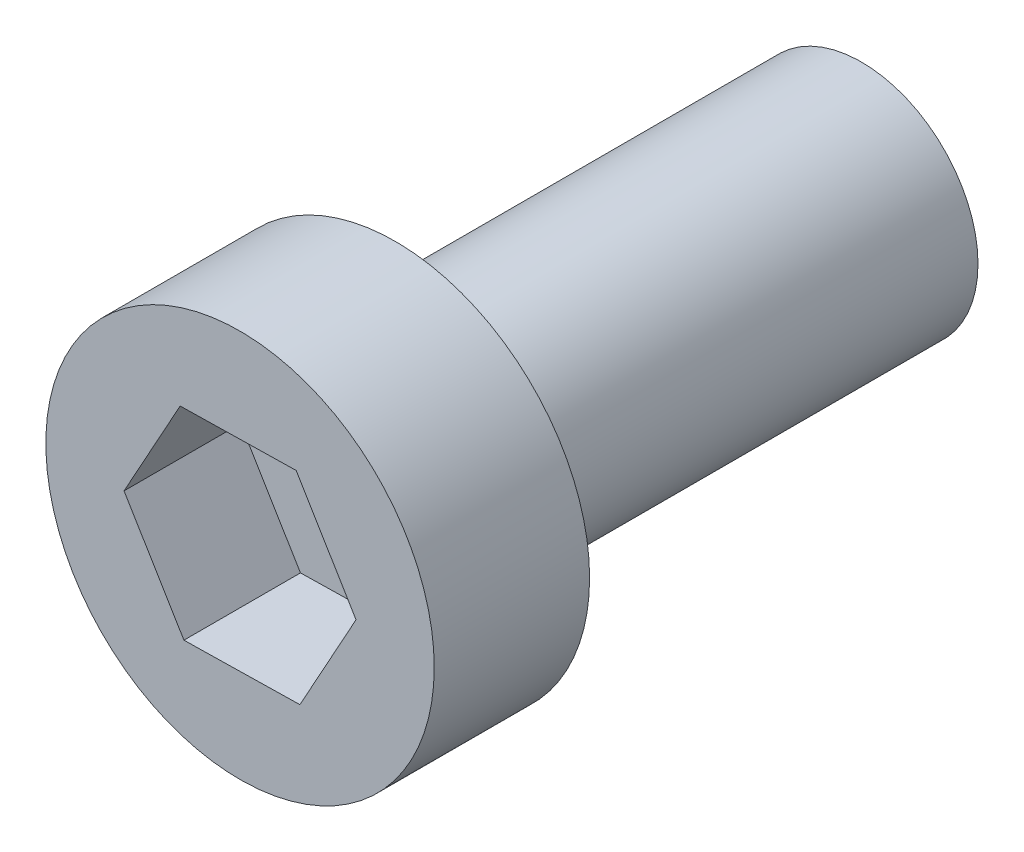
from build123d import *

# Parameters (mm, degrees)
SKETCH1_R           = 1.5
BOSS_EXTRUDE1_DEPTH = 6
SKETCH2_R           = 2.5
BOSS_EXTRUDE2_DEPTH = 2
CUT_EXTRUDE1_DEPTH  = 1.5


with BuildPart() as part:
    # Sketch1 → Boss-Extrude1 (new body)
    with BuildSketch(Plane.XY):
        Circle(SKETCH1_R)
    extrude(amount=-BOSS_EXTRUDE1_DEPTH)

    # Sketch2 → Boss-Extrude2 (add)
    with BuildSketch(Plane.XY):
        Circle(SKETCH2_R)
    extrude(amount=BOSS_EXTRUDE2_DEPTH)

    # Sketch3 → Cut-Extrude1 (cut)
    with BuildSketch(Plane.XY.offset(2)):
        Polygon((0.722266578, 1.307190321), (-0.770926737, 1.279096365), (-1.493193314, -0.028093956), (-0.722266578, -1.307190321), (0.770926737, -1.279096365), (1.493193314, 0.028093956), align=None)
    extrude(amount=-CUT_EXTRUDE1_DEPTH, mode=Mode.SUBTRACT)


solid = part.part
